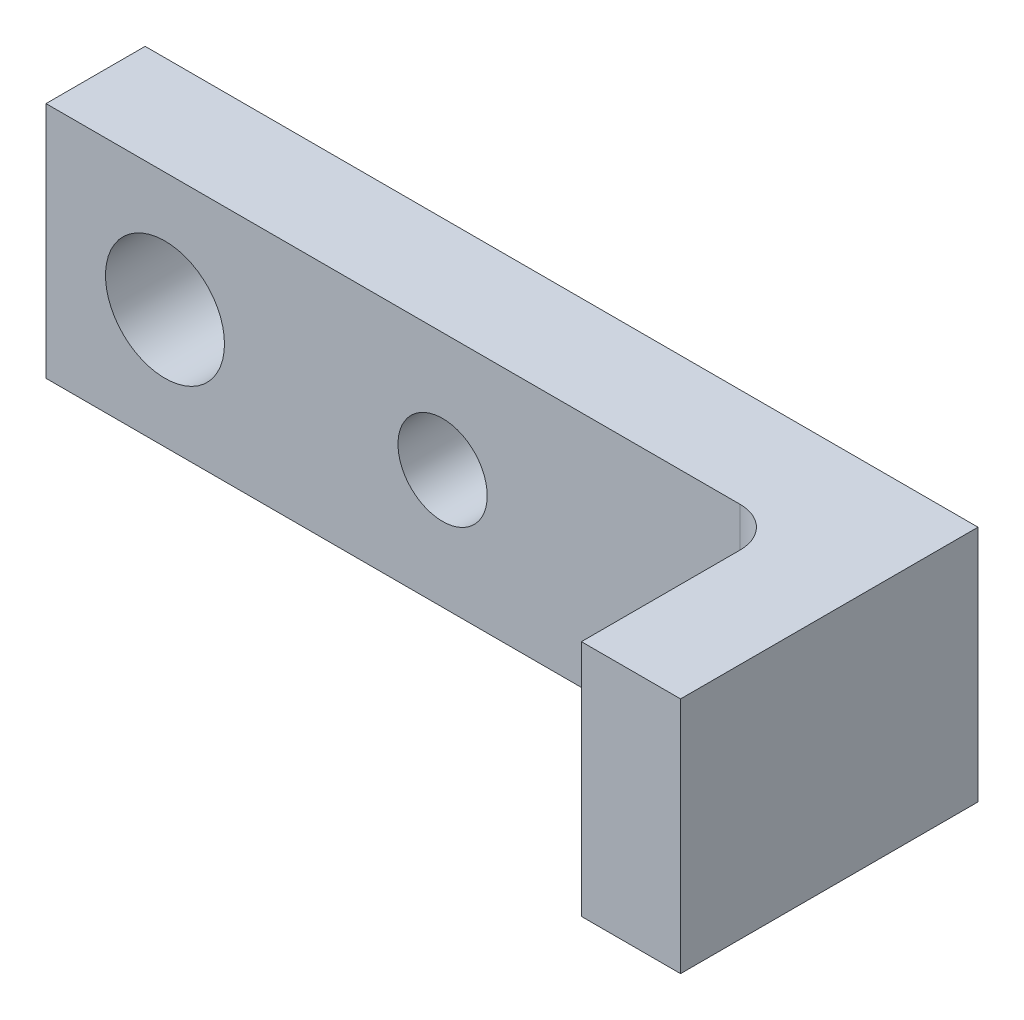
SolidWorks part; units mm, degrees
ref_plane "Front Plane" through (0, 0, 0) normal (0, 0, 1) x (1, 0, 0)
ref_plane "Top Plane" through (0, 0, 0) normal (0, 1, 0) x (1, 0, 0)
ref_plane "Right Plane" through (0, 0, 0) normal (1, 0, 0) x (0, 0, -1)
sketch "Sketch1" plane through (0, 0, 0) normal (0, 0, 1) x (1, 0, 0)
  line L0 (0, 6) -> (42, 6) construction
  line L1 (0, 0) -> (42, 0)
  line L2 (0, 0) -> (0, 12)
  line L3 (0, 12) -> (42, 12)
  line L4 (42, 0) -> (42, 12)
  circle A0 centre (20, 6) radius 2.25
  circle A1 centre (6, 6) radius 3
  dimension "D3" = 4.5
  dimension "D4" = 20
  dimension "D5" = 6
  dimension "D6" = 6
  dimension "D1" = 42
  dimension "D2" = 12
extrude "Boss-Extrude1" add sketch "Sketch1" along normal blind 5
sketch "Sketch2" plane through (0, 0, 5) normal (0, 0, 1) x (1, 0, 0)
  line L0 (42, 12) -> (0, 12) construction
  line L1 (42, 0) -> (37, 0)
  line L2 (42, 0) -> (42, 12)
  line L3 (42, 12) -> (37, 12)
  line L4 (37, 0) -> (37, 12)
  dimension "D1" = 5
extrude "Boss-Extrude2" add sketch "Sketch2" along normal blind 10
fillet "Fillet1" radius 2 1 edges at (37, 6, 5)
